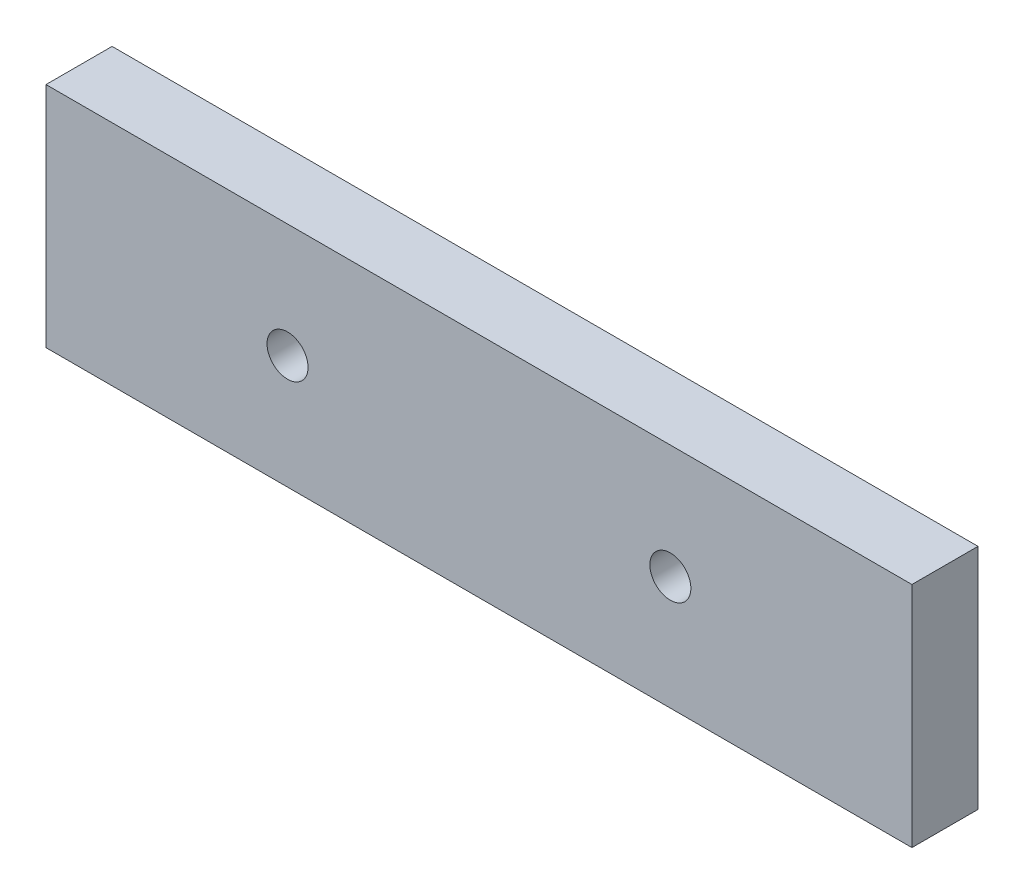
SolidWorks part; units mm, degrees
material "6061 合金"
ref_plane "前视基准面" through (0, 0, 0) normal (0, 0, 1) x (1, 0, 0)
ref_plane "上视基准面" through (0, 0, 0) normal (0, 1, 0) x (1, 0, 0)
ref_plane "右视基准面" through (0, 0, 0) normal (1, 0, 0) x (0, 0, -1)
sketch "草图1" plane through (0, 0, 0) normal (0, 0, 1) x (1, 0, 0)
  line L1 (-95, 25) -> (95, 25)
  line L2 (-95, 25) -> (-95, -25)
  line L3 (-95, -25) -> (95, -25)
  line L4 (95, 25) -> (95, -25)
  line L5 (-95, 25) -> (95, -25) construction
  line L6 (-95, -25) -> (95, 25) construction
  circle A0 centre (-42, 0) radius 4.5
  circle A1 centre (42, 0) radius 4.5
  point P0 (0, 0)
  dimension "D3" = 84
  dimension "D4" = 42
  dimension "D5" = 25
  dimension "D6" = 9
  dimension "D1" = 190
  dimension "D2" = 50
extrude "凸台-拉伸1" add sketch "草图1" along normal mid plane 14.5
